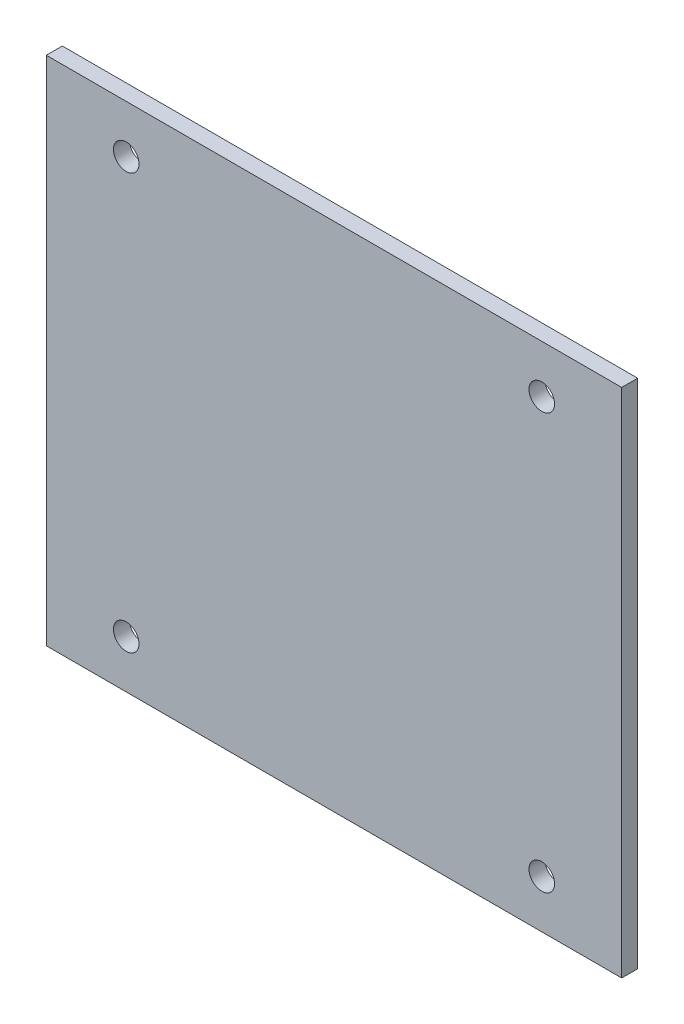
SolidWorks part; units mm, degrees
ref_plane "前视基准面" through (0, 0, 0) normal (0, 0, 1) x (1, 0, 0)
ref_plane "上视基准面" through (0, 0, 0) normal (0, 1, 0) x (1, 0, 0)
ref_plane "右视基准面" through (0, 0, 0) normal (1, 0, 0) x (0, 0, -1)
sketch "草图1" plane through (0, 0, 0) normal (0, 0, 1) x (1, 0, 0)
  line L1 (-90, -80) -> (90, -80)
  line L2 (-90, -80) -> (-90, 80)
  line L3 (-90, 80) -> (90, 80)
  line L4 (90, -80) -> (90, 80)
  line L5 (-90, -80) -> (90, 80) construction
  line L6 (-90, 80) -> (90, -80) construction
  point P0 (0, 0)
  dimension "D1" = 180
  dimension "D2" = 160
extrude "凸台-拉伸1" add sketch "草图1" along normal blind 5
sketch "草图2" plane through (0, 0, 5) normal (0, 0, 1) x (1, 0, 0)
  line L0 (0, 0) -> (0, 80) construction
  line L1 (90, 80) -> (-90, 80) construction
  line L2 (0, 0) -> (90, 0) construction
  line L3 (90, -80) -> (90, 80) construction
  circle A0 centre (-65, 65) radius 4
  circle A1 centre (65, 65) radius 4
  circle A2 centre (65, -65) radius 4
  circle A3 centre (-65, -65) radius 4
  dimension "D1" = 8
  dimension "D2" = 130
  dimension "D3" = 130
extrude "切除-拉伸1" cut sketch "草图2" against normal through all
